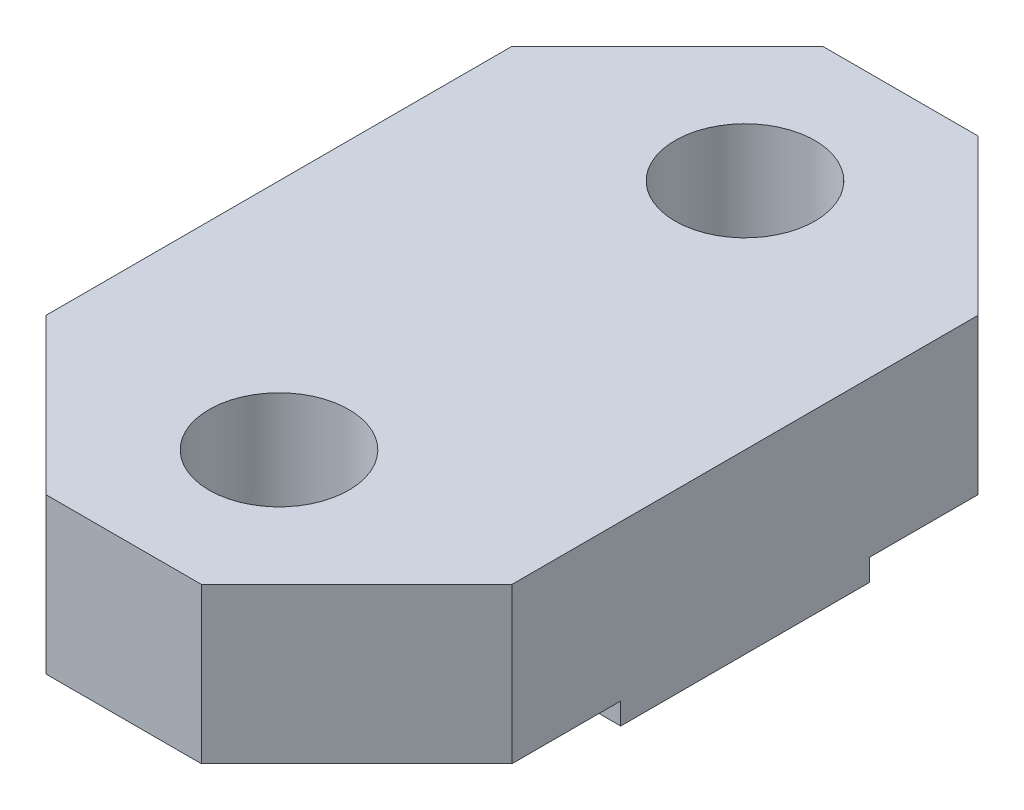
SolidWorks part; units mm, degrees
ref_plane "Front Plane" through (0, 0, 0) normal (0, 0, 1) x (1, 0, 0)
ref_plane "Top Plane" through (0, 0, 0) normal (0, 1, 0) x (1, 0, 0)
ref_plane "Right Plane" through (0, 0, 0) normal (1, 0, 0) x (0, 0, -1)
sketch "Sketch1" plane through (0, 0, 0) normal (0, 1, 0) x (1, 0, 0)
  line L1 (-7.5, -12.5) -> (7.5, -12.5)
  line L2 (-7.5, -12.5) -> (-7.5, 12.5)
  line L3 (-7.5, 12.5) -> (7.5, 12.5)
  line L4 (7.5, -12.5) -> (7.5, 12.5)
  line L5 (-7.5, -12.5) -> (7.5, 12.5) construction
  line L6 (-7.5, 12.5) -> (7.5, -12.5) construction
  point P0 (0, 0)
  dimension "D1" = 25
  dimension "D2" = 15
extrude "Boss-Extrude1" add sketch "Sketch1" along normal blind 5.7
sketch "Sketch2" plane through (0, 0, 0) normal (0, -1, 0) x (1, 0, 0)
  line L0 (7.5, 12.5) -> (7.5, -12.5) construction
  line L1 (-7.5, -12.5) -> (7.5, -12.5)
  line L2 (-7.5, -12.5) -> (-7.5, -4)
  line L3 (-7.5, -4) -> (7.5, -4)
  line L4 (7.5, -12.5) -> (7.5, -4)
  line L5 (0, 0) -> (-50000, 0) construction
  line L6 (-7.5, 4) -> (7.5, 4)
  line L7 (7.5, 12.5) -> (7.5, 4)
  line L8 (-7.5, 12.5) -> (7.5, 12.5)
  line L9 (-7.5, 12.5) -> (-7.5, 4)
  dimension "D1" = 8.5
extrude "Cut-Extrude1" cut sketch "Sketch2" against normal blind 0.7
chamfer "Chamfer1" distance 5 angle 45 4 edges at (7.5, 3.2, 12.5) (-7.5, 3.2, 12.5) (7.5, 3.2, -12.5) (-7.5, 3.2, -12.5)
hole_wizard "Ø4.5 (4.5) Diameter Hole1" positions "Sketch3" profile "Sketch4" hole size "Ø4.5" standard "GB" end condition through all
sketch "Sketch3" plane through (0, 5.7, 0) normal (0, 1, 0) x (1, 0, 0)
  line L0 (0, 0) -> (50000, 0) construction
  line L1 (7.5, -7.5) -> (7.5, 7.5) construction
  point P0 (0, 7.5)
  point P8 (7.5, 0)
  point P11 (0, -7.5)
  dimension "D1" = 15
sketch "Sketch4" plane through (0, 5.7, -7.5) normal (1, 0, 0) x (0, 0, 1)
  line L0 (0, 0) -> (0, 5.7)
  line L1 (0, 5.7) -> (2.25, 5.7)
  line L2 (2.25, 5.7) -> (2.25, 0)
  line L5 (2.25, 0) -> (0, 0)
  line L11 (0, -6.35) -> (0, 107.95) construction
  dimension "通孔孔直径" = 4.5
  dimension "通孔孔深度" = 5.7
